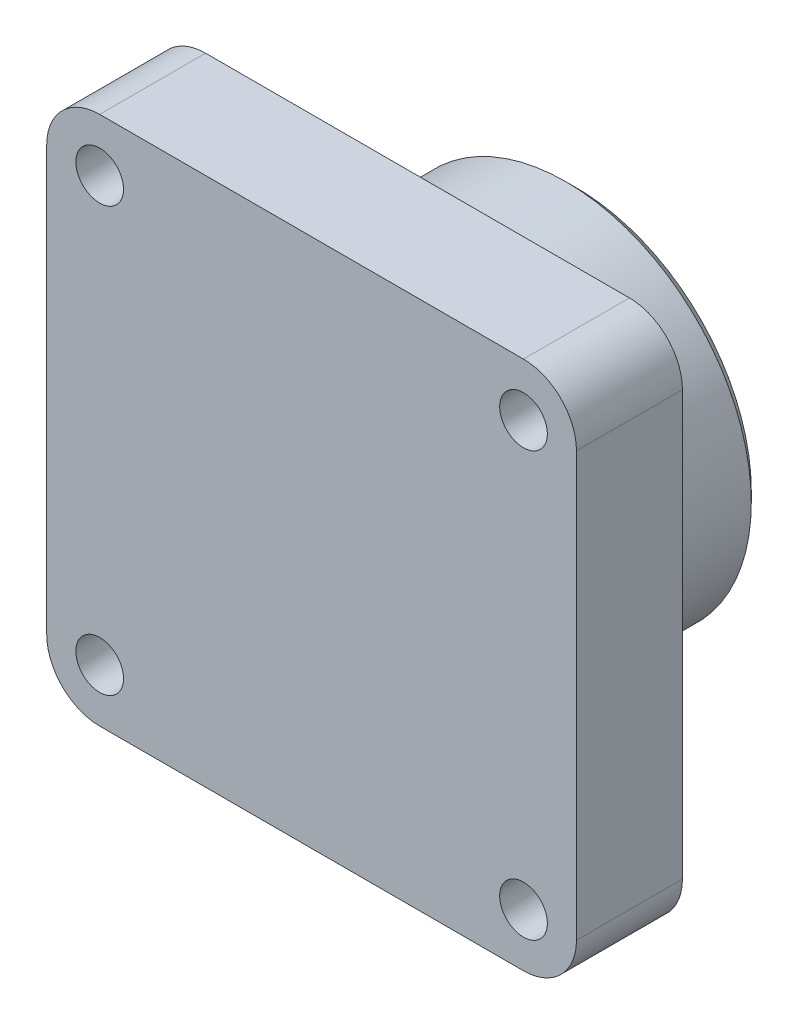
from build123d import *

# Parameters (mm, degrees)
SKETCH1_R           = 12.6
BOSS_EXTRUDE1_DEPTH = 10.8
SKETCH2_W           = 36
SKETCH2_H           = 36
BOSS_EXTRUDE2_DEPTH = 7.2
FILLET1_R           = 3.6
CHAMFER1_SIZE       = 0.72
SKETCH3_R           = 14.4
SKETCH3_R_2         = 12.6
CUT_EXTRUDE1_DEPTH  = 1.08
SKETCH4_W           = 1.08
SKETCH4_H           = 0.54
SKETCH5_R           = 1.62
CUT_EXTRUDE2_DEPTH  = 7.2
SKETCH6_R           = 8.1
CUT_EXTRUDE3_DEPTH  = 10.8


with BuildPart() as part:
    # Sketch1 → Boss-Extrude1 (new body)
    with BuildSketch(Plane.XY):
        with Locations(Location((0, 0, 0), (0, 0, 180))):
            Circle(SKETCH1_R)
    extrude(amount=BOSS_EXTRUDE1_DEPTH)

    # Sketch2 → Boss-Extrude2 (add)
    with BuildSketch(Plane.XY.offset(10.8)):
        Rectangle(SKETCH2_W, SKETCH2_H)
    extrude(amount=BOSS_EXTRUDE2_DEPTH)

    # Fillet1
    fillet1_edges = [part.edges().sort_by_distance(p)[0] for p in [
        (18, -18, 14.4),
        (18, 18, 14.4),
        (-18, 18, 14.4),
        (-18, -18, 14.4),
    ]]
    fillet(fillet1_edges, radius=FILLET1_R)

    # Chamfer1
    chamfer1_edges = [part.edges().sort_by_distance(p)[0] for p in [
        (12.6, 0, 0),
    ]]
    chamfer(chamfer1_edges, length=CHAMFER1_SIZE)

    # Sketch3 → Cut-Extrude1 (cut)
    with BuildSketch(Plane(origin=(0, 0, 10.8), x_dir=(-1, 0, 0), z_dir=(0, 0, -1))):
        Circle(SKETCH3_R)
        Circle(SKETCH3_R_2, mode=Mode.SUBTRACT)
    extrude(amount=-CUT_EXTRUDE1_DEPTH, mode=Mode.SUBTRACT)

    # Sketch4 → Cut-Revolve1 (revolve, cut)
    with BuildSketch(Plane(origin=(0, 0, 0), x_dir=(1, 0, 0), z_dir=(0, 1, 0)), mode=Mode.PRIVATE) as cut_revolve1_sk:
        with Locations((12.6, -6.3)):
            Rectangle(SKETCH4_W, SKETCH4_H)
    revolve(cut_revolve1_sk.sketch.rotate(Axis((0, 0, -2.746665179), (0, 0, 1)), 180), axis=Axis((0, 0, -2.746665179), (0, 0, 1)), mode=Mode.SUBTRACT)

    # Sketch5 → Cut-Extrude2 (cut)
    with BuildSketch(Plane(origin=(0, 0, 10.8), x_dir=(-1, 0, 0), z_dir=(0, 0, -1))):
        with Locations((14.4, 14.4)):
            Circle(SKETCH5_R)
        with Locations((14.4, -14.4)):
            Circle(SKETCH5_R)
        with Locations((-14.4, -14.4)):
            Circle(SKETCH5_R)
        with Locations((-14.4, 14.4)):
            Circle(SKETCH5_R)
    extrude(amount=-CUT_EXTRUDE2_DEPTH, mode=Mode.SUBTRACT)

    # Sketch6 → Cut-Extrude3 (cut)
    with BuildSketch(Plane(origin=(0, 0, 0), x_dir=(-1, 0, 0), z_dir=(0, 0, -1))):
        Circle(SKETCH6_R)
    extrude(amount=-CUT_EXTRUDE3_DEPTH, mode=Mode.SUBTRACT)


solid = part.part
